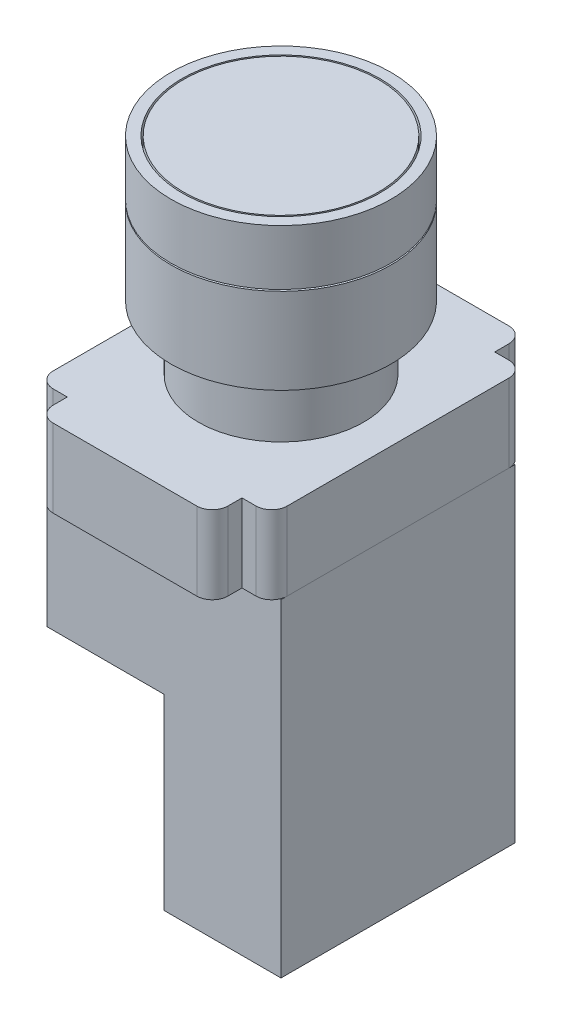
SolidWorks part; units mm, degrees
ref_plane "前视基准面" through (0, 0, 0) normal (0, 0, 1) x (1, 0, 0)
ref_plane "上视基准面" through (0, 0, 0) normal (0, 1, 0) x (1, 0, 0)
ref_plane "右视基准面" through (0, 0, 0) normal (1, 0, 0) x (0, 0, -1)
sketch "草图1" plane through (0, 0, 0) normal (0, 0, 1) x (1, 0, 0)
  line L0 (0, 0) -> (0, 19.2) construction
  line L1 (12.5, 19.2) -> (14.1, 19.2)
  line L2 (14.1, 19.2) -> (14.1, 8.2)
  line L3 (14.1, 8.2) -> (10.6, 8.2)
  line L4 (10.6, 8.2) -> (10.6, 0)
  line L5 (10.6, 0) -> (0, 0)
  line L6 (0, 0) -> (0, 19.2)
  line L9 (0, 19.2) -> (0, 26.5)
  line L10 (0, 26.5) -> (12.5, 26.5)
  line L11 (12.5, 19.2) -> (12.5, 26.5)
  dimension "D1" = 21.2
  dimension "D2" = 28.2
  dimension "D3" = 8.2
  dimension "D4" = 19.2
  dimension "D5" = 12.5
  dimension "D6" = 26.5
revolve "旋转1" add sketch "草图1" angle 360 about L0
sketch "草图2" plane through (0, 0, 0) normal (0, -1, 0) x (1, 0, 0)
  line L0 (15, -20) -> (-15, 20) construction
  line L1 (15, 20) -> (-15, 20)
  line L2 (15, 20) -> (15, -20)
  line L3 (15, -20) -> (-15, -20)
  line L4 (-15, 20) -> (-15, -20)
  dimension "D1" = 30
  dimension "D2" = 40
extrude "拉伸1" add sketch "草图2" along normal blind 10 separate body
sketch "草图3" plane through (0, -10, 0) normal (0, -1, 0) x (1, 0, 0)
  line L0 (15, -20) -> (15, 20) construction
  line L1 (15, 15) -> (0, 15)
  line L2 (15, 15) -> (15, -15)
  line L3 (15, -15) -> (0, -15)
  line L4 (0, 15) -> (0, -15)
  dimension "D1" = 30
extrude "拉伸2" add sketch "草图3" along normal blind 42 separate body
sketch "草图7" plane through (0, 0, 0) normal (0, 1, 0) x (-1, 0, 0)
  line L0 (0, 20) -> (0, -20) construction
  line L1 (-15, 20) -> (-11.2, 20)
  line L2 (-15, 20) -> (-15, 16.2)
  line L3 (-15, 16.2) -> (-11.2, 16.2)
  line L4 (-11.2, 20) -> (-11.2, 16.2)
  line L5 (-15, 20) -> (15, 20) construction
  line L6 (15, -20) -> (-15, -20) construction
  line L7 (-15, 0) -> (15, 0) construction
  line L8 (-15, -20) -> (-15, 20) construction
  line L9 (15, 20) -> (15, -20) construction
  line L10 (11.2, 20) -> (11.2, 16.2)
  line L11 (15, 16.2) -> (11.2, 16.2)
  line L12 (15, 20) -> (15, 16.2)
  line L13 (15, 20) -> (11.2, 20)
  line L14 (15, -20) -> (11.2, -20)
  line L15 (15, -20) -> (15, -16.2)
  line L16 (15, -16.2) -> (11.2, -16.2)
  line L17 (11.2, -20) -> (11.2, -16.2)
  line L18 (-11.2, -20) -> (-11.2, -16.2)
  line L19 (-15, -16.2) -> (-11.2, -16.2)
  line L20 (-15, -20) -> (-15, -16.2)
  line L21 (-15, -20) -> (-11.2, -20)
  dimension "D1" = 3.8
extrude "切除-拉伸2" cut sketch "草图7" against normal up to next (10 mm away)
fillet "圆角1" radius 2 8 edges at (-15, -5, 16.2) (-11.2, -5, 20) (11.2, -5, 20) (15, -5, 16.2) (15, -5, -16.2) (11.2, -5, -20) (-11.2, -5, -20) (-15, -5, -16.2)
sketch "草图8" plane through (0, -10, 0) normal (0, 1, 0) x (-1, 0, 0)
  line L0 (0, 15) -> (0, -15) construction
  line L1 (0, -15) -> (15, -15)
  line L2 (0, -15) -> (0, 15)
  line L3 (0, 15) -> (15, 15)
  line L4 (15, -15) -> (15, 15)
  line L5 (-15, 15) -> (0, 15) construction
extrude "拉伸3" add sketch "草图8" against normal blind 18
sketch "草图11" plane through (0, 0, 0) normal (0, 0, 1) x (1, 0, 0)
  line L0 (0, 0) -> (0, 26.5) construction
  line L1 (14.1, 26.5) -> (12.7, 26.5)
  line L2 (14.1, 26.5) -> (14.1, 19.4)
  line L3 (14.1, 19.4) -> (12.7, 19.4)
  line L4 (12.7, 19.4) -> (12.7, 26.5)
  line L5 (-14.1, 8.2) -> (14.1, 8.2) construction
  line L7 (14.1, 19.2) -> (-14.1, 19.2) construction
  line L8 (12.5, 19.2) -> (12.5, 26.5) construction
  line L10 (14.1, 8.2) -> (14.1, 19.2) construction
  dimension "D1" = 0.2
  dimension "D2" = 0.2
  dimension "D3" = 18.3
revolve "旋转2" add sketch "草图11" angle 360 about L0
